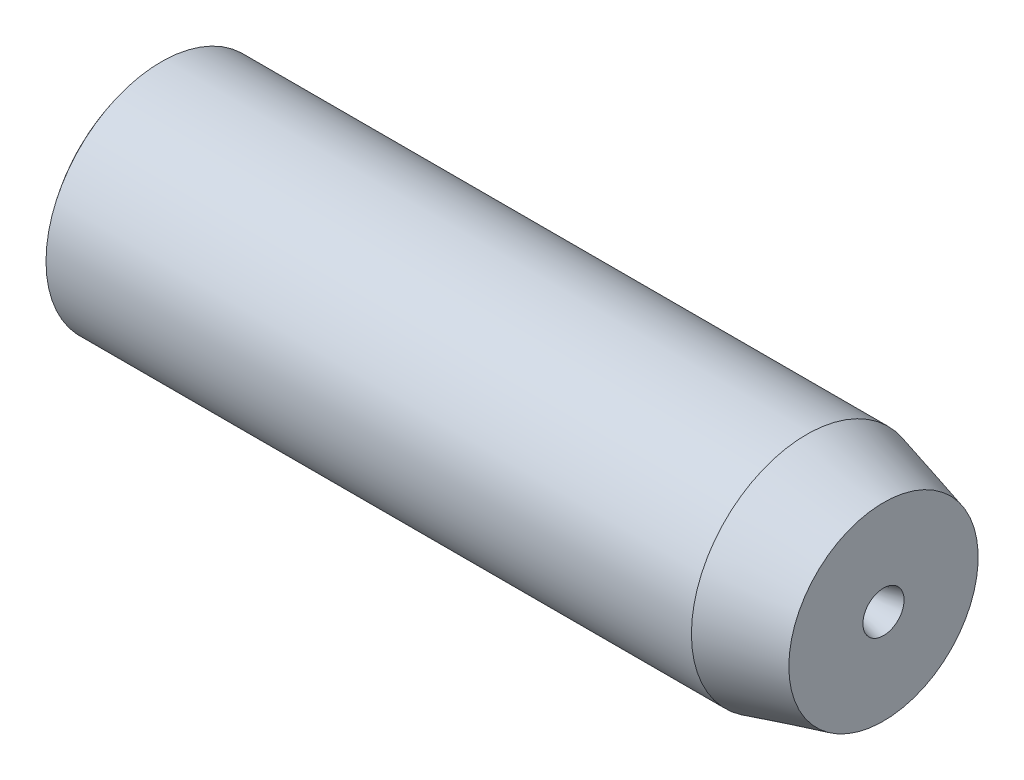
from build123d import *


with BuildPart() as part:
    # 草图1 → 旋转1 (revolve)
    with BuildSketch(Plane.XY, mode=Mode.PRIVATE) as revolve_1_sk:
        with BuildLine():
            Line((-8.8, 3), (8, 3))
            Line((8, 3), (10, 2.464101615))
            Line((10, 2.464101615), (10, 0))
            Line((10, 0), (-10, 0))
            ThreePointArc((-10, 0), (-9.605742928, 1.582297171), (-8.8, 3))
        make_face()
    revolve(revolve_1_sk.sketch.rotate(Axis((10, 0, 0), (-1, 0, 0)), 270), axis=Axis((10, 0, 0), (-1, 0, 0)))

    # 草图2 → 切除-旋转1 (revolve, cut)
    with BuildSketch(Plane.XY, mode=Mode.PRIVATE) as cut_revolve_1_sk:
        Polygon((8, 0), (12, 1.07179677), (12, 0), align=None)
    revolve(cut_revolve_1_sk.sketch.rotate(Axis((12, 0, 0), (-1, 0, 0)), 90), axis=Axis((12, 0, 0), (-1, 0, 0)), mode=Mode.SUBTRACT)


solid = part.part
